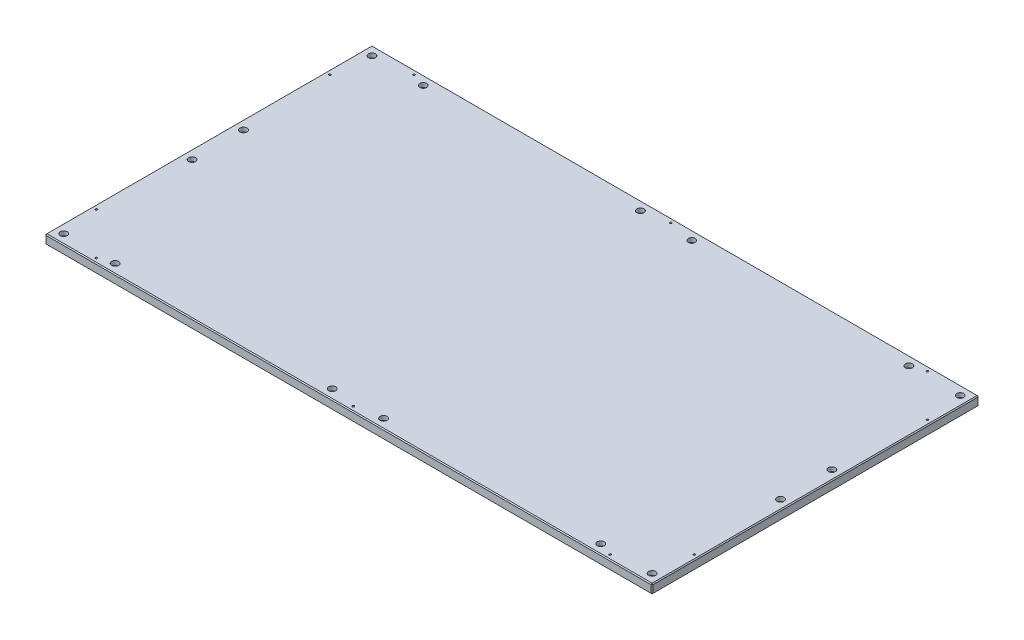
SolidWorks part; units mm, degrees
material "普通碳钢"
ref_plane "前视基准面" through (0, 0, 0) normal (0, 0, 1) x (1, 0, 0)
ref_plane "上视基准面" through (0, 0, 0) normal (0, 1, 0) x (1, 0, 0)
ref_plane "右视基准面" through (0, 0, 0) normal (1, 0, 0) x (0, 0, -1)
sketch "草图1" plane through (0, 0, 0) normal (0, 1, 0) x (1, 0, 0)
  line L0 (-102.6874, 0) -> (127.2051, 0) construction
  line L1 (0, 74.086) -> (0, -85.1742) construction
  line L3 (-650, 350) -> (650, 350)
  line L4 (-650, 350) -> (-650, -350)
  line L5 (-650, -350) -> (650, -350)
  line L6 (650, 350) -> (650, -350)
  dimension "D1" = 1300
  dimension "D2" = 700
extrude "凸台-拉伸1" add sketch "草图1" along normal mid plane 20
chamfer "倒角1" distance 2 angle 45 12 edges at (-650, 0, 350) (-650, 0, -350) (0, -10, 350) (-650, -10, 0) (0, -10, -350) (0, 10, -350) (-650, 10, 0) (0, 10, 350) (650, 0, 350) (650, 10, 0) (650, 0, -350) (650, -10, 0)
hole_wizard "打孔尺寸根据内六角圆柱头螺钉的类型1" positions "3D草图1" profile "草图2" counterbore size "M8" standard "Gb" end condition through all
sketch3d "3D草图1"
  point P0 (630, 10, -330)
  dimension "D1" = 630
  dimension "D2" = 20
sketch "草图2" plane through (630, 10, -330) normal (1, 0, 0) x (0, 0, 1)
  line L0 (0, 0) -> (0, 20)
  line L1 (0, 20) -> (4.5, 20)
  line L3 (4.5, 20) -> (4.5, 9)
  line L4 (4.5, 9) -> (7.5, 9)
  line L5 (7.5, 9) -> (7.5, 0)
  line L7 (7.5, 0) -> (0, 0)
  line L11 (0, -6.35) -> (0, 107.95) construction
  dimension "通孔孔直径" = 9
  dimension "通孔孔深度" = 20
  dimension "柱形沉头孔直径" = 15
  dimension "柱形沉头孔深度" = 9
pattern_linear "阵列(线性)1" count 2 spacing 110 along (-1, 0, 0) of "打孔尺寸根据内六角圆柱头螺钉的类型1"
hole_wizard "打孔尺寸根据内六角圆柱头螺钉的类型2" positions "3D草图2" profile "草图3" counterbore size "M8" standard "Gb" end condition through all
sketch3d "3D草图2"
  point P0 (630, 10, -55)
  dimension "D1" = 55
  dimension "D2" = 20
sketch "草图3" plane through (630, 10, -55) normal (1, 0, 0) x (0, 0, 1)
  line L0 (0, 0) -> (0, 20)
  line L1 (0, 20) -> (4.5, 20)
  line L3 (4.5, 20) -> (4.5, 9)
  line L4 (4.5, 9) -> (7.5, 9)
  line L5 (7.5, 9) -> (7.5, 0)
  line L7 (7.5, 0) -> (0, 0)
  line L11 (0, -6.35) -> (0, 107.95) construction
  dimension "通孔孔直径" = 9
  dimension "通孔孔深度" = 20
  dimension "柱形沉头孔直径" = 15
  dimension "柱形沉头孔深度" = 9
pattern_linear "阵列(线性)2" count 2 spacing 110 along (0, 0, 1) of "打孔尺寸根据内六角圆柱头螺钉的类型2"
mirror "镜向1" about plane through (0, 0, 0) normal (1, 0, 0) of "打孔尺寸根据内六角圆柱头螺钉的类型2", "阵列(线性)2"
mirror "镜向2" about plane through (0, 0, 0) normal (0, 0, 1) of "阵列(线性)1", "打孔尺寸根据内六角圆柱头螺钉的类型1"
pattern_linear "阵列(线性)3" count 3 spacing 575 along (-1, 0, 0) of "打孔尺寸根据内六角圆柱头螺钉的类型1", "阵列(线性)1", "镜向2"
hole_wizard "M5 螺纹孔1" positions "3D草图3" profile "草图14" tap size "M5" standard "Gb"
sketch3d "3D草图3"
  point P0 (550, 10, -340)
  dimension "D1" = 550
  dimension "D2" = 10
sketch "草图14" plane through (550, 10, -340) normal (1, 0, 0) x (0, 0, 1)
  line L0 (0, 0) -> (0, 23.6618)
  line L1 (0, 23.6618) -> (2.1, 22.4)
  line L2 (2.1, 22.4) -> (2.1, 0)
  line L5 (2.1, 0) -> (0, 0)
  line L10 (0, 23.6618) -> (-2.1, 22.4) construction
  line L11 (0, -6.35) -> (0, 107.95) construction
  dimension "螺纹孔钻头直径" = 4.2
  dimension "螺纹孔钻头深度" = 22.4
  dimension "导头角度" = 118
pattern_linear "阵列(线性)4" count 3 spacing 550 along (-1, 0, 0) of "M5 螺纹孔1"
mirror "镜向3" about plane through (0, 0, 0) normal (0, 0, 1) of "M5 螺纹孔1", "阵列(线性)4"
hole_wizard "M5 螺纹孔2" positions "3D草图4" profile "草图15" tap size "M5" standard "Gb"
sketch3d "3D草图4"
  point P0 (-640, 10, -250)
  dimension "D1" = 250
  dimension "D2" = 10
sketch "草图15" plane through (-640, 10, -250) normal (1, 0, 0) x (0, 0, 1)
  line L0 (0, 0) -> (0, 23.6618)
  line L1 (0, 23.6618) -> (2.1, 22.4)
  line L2 (2.1, 22.4) -> (2.1, 0)
  line L5 (2.1, 0) -> (0, 0)
  line L10 (0, 23.6618) -> (-2.1, 22.4) construction
  line L11 (0, -6.35) -> (0, 107.95) construction
  dimension "螺纹孔钻头直径" = 4.2
  dimension "螺纹孔钻头深度" = 22.4
  dimension "导头角度" = 118
mirror "镜向4" about plane through (0, 0, 0) normal (0, 0, 1) of "M5 螺纹孔2"
mirror "镜向5" about plane through (0, 0, 0) normal (1, 0, 0) of "镜向4", "M5 螺纹孔2"
